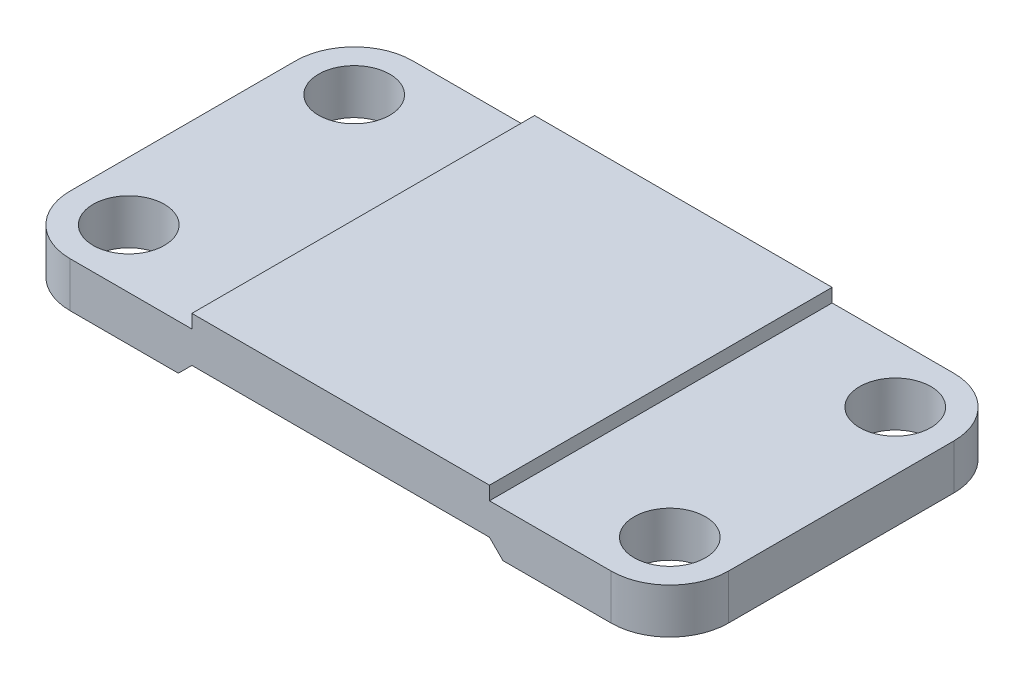
from build123d import *

# Parameters (mm, degrees)
SKETCH1_R           = 200.720721903
BOSS_EXTRUDE1_DEPTH = 330.2
SKETCH3_W           = 1676.4
SKETCH3_H           = 1930.4
BOSS_EXTRUDE4_DEPTH = 76.2
CUT_EXTRUDE2_DEPTH  = 76.2
CUT_EXTRUDE6_DEPTH  = 2708.334992202


with BuildPart() as part:
    # Sketch1 → Boss-Extrude1 (new body)
    with BuildSketch(Plane(origin=(0, 0, 0), x_dir=(1, 0, 0), z_dir=(0, 1, 0))):
        with BuildLine():
            Line((1524, 965.2), (-1524, 965.2))
            ThreePointArc((-1524, 965.2), (-1757.486659148, 868.486659148), (-1854.2, 635))
            Line((-1854.2, 635), (-1854.2, -635))
            ThreePointArc((-1854.2, -635), (-1757.486659148, -868.486659148), (-1524, -965.2))
            Line((-1524, -965.2), (1524, -965.2))
            ThreePointArc((1524, -965.2), (1757.486659148, -868.486659148), (1854.2, -635))
            Line((1854.2, -635), (1854.2, 635))
            ThreePointArc((1854.2, 635), (1757.486659148, 868.486659148), (1524, 965.2))
        make_face()
        with Locations(Location((-1524, 635, 0), (0, 0, 270))):
            Circle(SKETCH1_R, mode=Mode.SUBTRACT)
        with Locations(Location((1524, 635, 0), (0, 0, 270))):
            Circle(SKETCH1_R, mode=Mode.SUBTRACT)
        with Locations(Location((1524, -635, 0), (0, 0, 270))):
            Circle(SKETCH1_R, mode=Mode.SUBTRACT)
        with Locations(Location((-1524, -635, 0), (0, 0, 270))):
            Circle(SKETCH1_R, mode=Mode.SUBTRACT)
    extrude(amount=BOSS_EXTRUDE1_DEPTH)

    # Sketch3 → Boss-Extrude4 (add)
    with BuildSketch(Plane(origin=(0, 330.2, 0), x_dir=(1, 0, 0), z_dir=(0, 1, 0))):
        Rectangle(SKETCH3_W, SKETCH3_H)
    extrude(amount=BOSS_EXTRUDE4_DEPTH)

    # Sketch5 → Cut-Extrude2 (cut)
    with BuildSketch(Plane.XZ):
        with BuildLine():
            Line((-1524, -965.2), (1524, -965.2))
            ThreePointArc((1524, -965.2), (1757.486659148, -868.486659148), (1854.2, -635))
            Line((1854.2, -635), (1854.2, 635))
            ThreePointArc((1854.2, 635), (1757.486659148, 868.486659148), (1524, 965.2))
            Line((1524, 965.2), (-1524, 965.2))
            ThreePointArc((-1524, 965.2), (-1757.486659148, 868.486659148), (-1854.2, 635))
            Line((-1854.2, 635), (-1854.2, -635))
            ThreePointArc((-1854.2, -635), (-1757.486659148, -868.486659148), (-1524, -965.2))
        make_face()
    extrude(amount=-CUT_EXTRUDE2_DEPTH, mode=Mode.SUBTRACT)

    # Sketch6 → Cut-Extrude6 (cut, through all)
    with BuildSketch(Plane.XY.offset(965.2)):
        Polygon((-914.4, 76.2), (914.4, 76.2), (838.2, 152.4), (-838.2, 152.4), align=None)
    extrude(amount=-CUT_EXTRUDE6_DEPTH, mode=Mode.SUBTRACT)


solid = part.part
